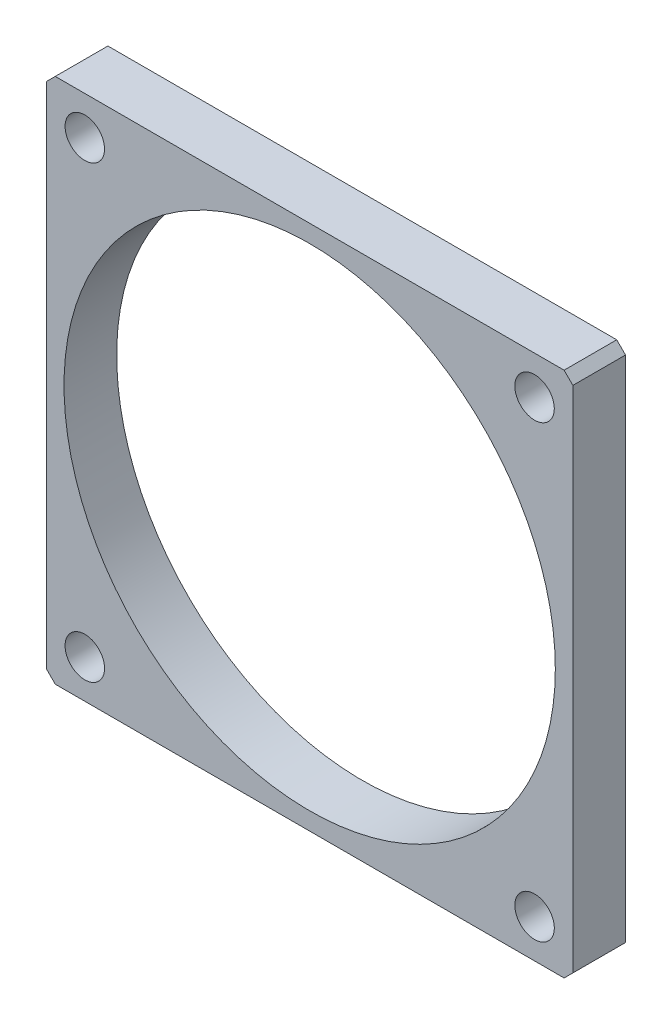
from build123d import *

# Parameters (mm, degrees)
SKETCH1_W           = 120
SKETCH1_H           = 120
BOSS_EXTRUDE1_DEPTH = 12
SKETCH2_R           = 56
CUT_EXTRUDE1_DEPTH  = 86.697141143
CIRPATTERN1_COUNT   = 4
CHAMFER1_SIZE       = 2


with BuildPart() as part:
    # Sketch1 → Boss-Extrude1 (new body)
    with BuildSketch(Plane.XY):
        Rectangle(SKETCH1_W, SKETCH1_H)
    extrude(amount=BOSS_EXTRUDE1_DEPTH)

    # Sketch2 → Cut-Extrude1 (cut, through all)
    with BuildSketch(Plane.XY.offset(12)):
        Circle(SKETCH2_R)
    extrude(amount=-CUT_EXTRUDE1_DEPTH, mode=Mode.SUBTRACT)

    # Sketch3 → M8 Clearance Hole1 (revolve, cut)
    with BuildSketch(Plane(origin=(-51.265241636, 51.265241636, 12), x_dir=(0, -1, 0), z_dir=(1, 0, 0))):
        Polygon((0, 0), (0, 52.703872786), (4.5, 50), (4.5, 0), align=None)
    m8_clearance_hole1 = revolve(axis=Axis((-51.265241636, 51.265241636, 18.35), (0, 0, -1)), mode=Mode.SUBTRACT)

    # CirPattern1: M8 Clearance Hole1 ×4 about axis
    cirpattern1_axis = Axis((0, 0, 0), (0, 0, 1))
    for i in range(1, CIRPATTERN1_COUNT):
        add(m8_clearance_hole1.rotate(cirpattern1_axis, i * 360 / CIRPATTERN1_COUNT), mode=Mode.SUBTRACT)

    # Chamfer1
    chamfer1_edges = [part.edges().sort_by_distance(p)[0] for p in [
        (60, -60, 6),
        (-60, -60, 6),
        (-60, 60, 6),
        (60, 60, 6),
    ]]
    chamfer(chamfer1_edges, length=CHAMFER1_SIZE)


solid = part.part
